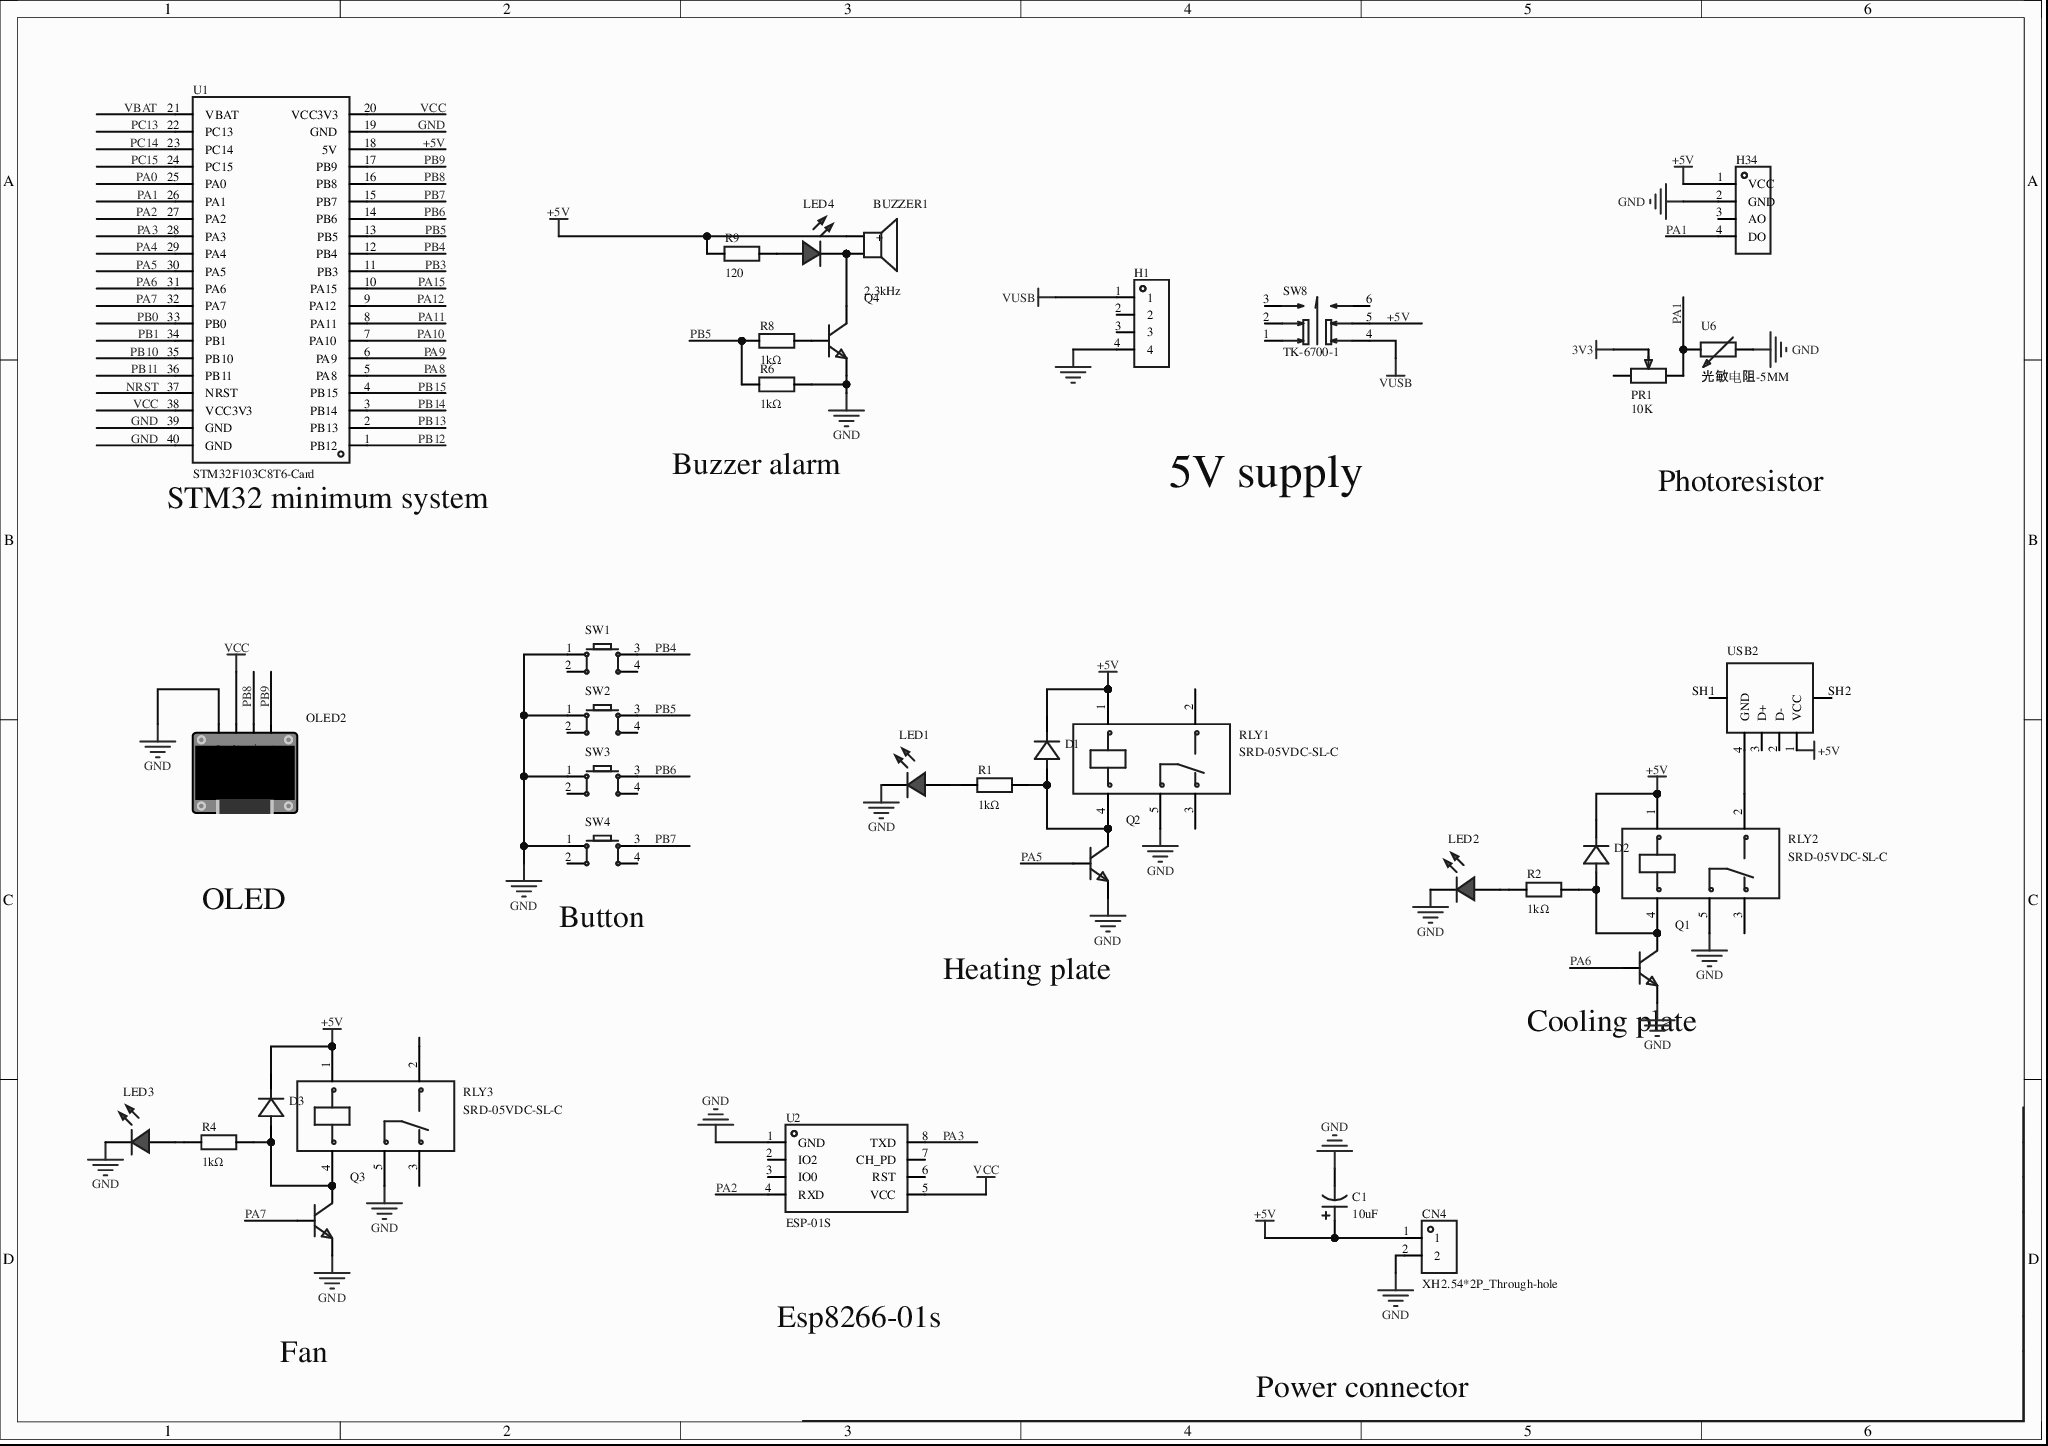
[diagram p0: MISC51908-3.schdoc]
# Altium project MISC51908-2.PrjPcb
1 sheet, 36 parts. Net scope: global (net labels, ports and power ports of the same name join across sheets).
Board file: MISC51908.pcbdoc

## Sheet MISC51908-3.schdoc
size 297 x 209 mm; Version: V1.0; @Project Name: MISC51908; @Page Count: 1; @Update Date: 2026-05-05; @Create Date: 2026-05-05; @Schematic Name: MISC51908; @Page No: 1; @Create Time: 23:22:16; @Update Time: 17:32:40; @Board Name: MISC51908

### Parts
BUZZER1  2.3kHz  [BUZ-TH_BD12.0-P7.60-D0.6-FD]
C1  10uF  [CAP-TH_BD5.0-P2.00-D0.8-FD-10UF50VC110GL]
CN4  XH2.54*2P_Through-hole  [CONN-TH_2P-P2.50-XH2.54-2P]
D1  (no value)  [DO_1N4007]
D2  (no value)  [DO_1N4007]
D3  (no value)  [DO_1N4007]
H1  (no value)  [HDR-TH_4P-P2.54-V-F]
H34  (no value)  [HDR-TH_4P-P2.54-V-F]
LED1  (no value)  [LED_TH-3mm]
LED2  (no value)  [LED_TH-3mm]
LED3  (no value)  [LED_TH-3mm]
LED4  (no value)  [LED_TH-3mm]
OLED2  (no value)  [0.96OLED_4P]
PR1  10K  [R_3386P]
Q1  (no value)  [S8050_TO_92]
Q2  (no value)  [S8050_TO_92]
Q3  (no value)  [S8050_TO_92]
Q4  (no value)  [S8050_TO_92]
R1  1kΩ  [Res_1/4W]
R2  1kΩ  [Res_1/4W]
R4  1kΩ  [Res_1/4W]
R6  1kΩ  [Res_1/4W]
R8  1kΩ  [Res_1/4W]
R9  120  [Res_1/4W]
RLY1  SRD-05VDC-SL-C  [RELAY-TH_SRD-XXVDC-XL-C]
RLY2  SRD-05VDC-SL-C  [RELAY-TH_SRD-XXVDC-XL-C]
RLY3  SRD-05VDC-SL-C  [RELAY-TH_SRD-XXVDC-XL-C]
SW1  (no value)  [SW-TH_4P-L6.0-W6.0-P4.50-LS6.5]
SW2  (no value)  [SW-TH_4P-L6.0-W6.0-P4.50-LS6.5]
SW3  (no value)  [SW-TH_4P-L6.0-W6.0-P4.50-LS6.5]
SW4  (no value)  [SW-TH_4P-L6.0-W6.0-P4.50-LS6.5]
SW8  TK-6700-1  [SW-TH_TK-6700-1]
U1  STM32F103C8T6-Card  [CONN-TH_L53.3-W22.9_STM32F103C8T6-CARD]
U2  ESP-01S  [WIFIM-TH_ESP-01S]
U6  光敏电阻-5MM  [RES-TH_L4.9-W4.3-P3.4]
USB2  (no value)  [USB_ Type-A]

### Nets
3V3: PR1.2
+5V: BUZZER1.1(+) C1.1 CN4.1 D1.1(K) D2.1(K) D3.1(K) H34.1(VCC) R9.1 RLY1.1 RLY2.1 RLY3.1 SW8.5 U1.18(5V) USB2.1(VCC)
GND: C1.2 CN4.2 H1.4 H34.2(GND) LED1.2(A) LED2.2(A) LED3.2(A) OLED2.1(GND) Q1.1(E) Q2.1(E) Q3.1(E) Q4.1(E) R6.2 RLY1.5 RLY2.5 RLY3.5 SW1.1 SW2.1 SW3.1 SW4.1 U1.19(GND) U1.39(GND) U1.40(GND) U2.1(GND) U6.1
VCC: OLED2.2(VCC) U1.20(VCC3V3) U1.38(VCC3V3) U2.5(VCC)
VUSB: H1.1 SW8.4
NRST: U1.37(NRST)
PA0: U1.25(PA0)
PA1: H34.4(DO) PR1.1 U1.26(PA1) U6.2
PA2: U1.27(PA2) U2.4(RXD)
PA3: U1.28(PA3) U2.8(TXD)
PA4: U1.29(PA4)
PA5: Q2.2(B) U1.30(PA5)
PA6: Q1.2(B) U1.31(PA6)
PA7: Q3.2(B) U1.32(PA7)
PA8: U1.5(PA8)
PA9: U1.6(PA9)
PA10: U1.7(PA10)
PA11: U1.8(PA11)
PA12: U1.9(PA12)
PA15: U1.10(PA15)
PB0: U1.33(PB0)
PB1: U1.34(PB1)
PB3: U1.11(PB3)
PB4: SW1.3 U1.12(PB4)
PB5: R6.1 R8.1 SW2.3 U1.13(PB5)
PB6: SW3.3 U1.14(PB6)
PB7: SW4.3 U1.15(PB7)
PB8: OLED2.3(SCL) U1.16(PB8)
PB9: OLED2.4(SDA) U1.17(PB9)
PB10: U1.35(PB10)
PB11: U1.36(PB11)
PB12: U1.1(PB12)
PB13: U1.2(PB13)
PB14: U1.3(PB14)
PB15: U1.4(PB15)
PC13: U1.22(PC13)
PC14: U1.23(PC14)
PC15: U1.24(PC15)
VBAT: U1.21(VBAT)
NetBUZZER1_2: BUZZER1.2 LED4.2(A) Q4.3(C)
NetD1_2: D1.2(A) Q2.3(C) R1.2 RLY1.4
NetD2_2: D2.2(A) Q1.3(C) R2.2 RLY2.4
NetD3_2: D3.2(A) Q3.3(C) R4.2 RLY3.4
NetLED1_1: LED1.1(C) R1.1
NetLED2_1: LED2.1(C) R2.1
NetLED3_1: LED3.1(C) R4.1
NetLED4_1: LED4.1(C) R9.2
NetQ4_2: Q4.2(B) R8.2
NetRLY2_2: RLY2.2 USB2.4(GND)

Not connected (* = marked no-connect by the designer): H1 2 3; H34 3(AO); PR1 3; RLY1 2 3; RLY2 3; RLY3 2 3; SW1 2 4; SW2 2 4; SW3 2 4; SW4 2 4; SW8 1* 2* 3* 6*; U2 2(IO2)* 3(IO0)* 6(RST)* 7(CH_PD)*; USB2 2(D-) 3(D+) SH1 SH2

### Notes on the sheet
- (near U1) STM32 minimum system
- Buzzer alarm
- 5V supply
- Photoresistor
- OLED
- (near SW4) Button
- Heating plate
- (near Q1) Cooling plate
- Fan
- Esp8266-01s
- Power connector

### Library data of the parts
BUZZER1 = TMB12A05_C96093: Drive mode:Active (built-in driver circuit);Construction type:Electromagnetic;Rated voltage:5V;Frequency:2.3kHz;Sound pressure (SPL):85dB@5V,10cm;; Manufacturer: 华能; 3D Model: 16ab50e14c5b4f2c986c135bdba60e37; 3D Model Transform: 472.44,472.176,0,90,0,0,-0.787,0,-177.165; Rated Voltage: 5V; Operating Voltage: 4V~8V; AddInBom: yes; ModelName: BUZ-TH_D12.0-H9.5-P7.60; Symbol: TMB12A05; Device: TMB12A05_C96093; LCSC Part Name: TMB12A05; Supplier Part: C96093; Manufacturer Part: TMB12A05; Supplier Footprint: 插件,D=12mm; JLCPCB Part Class: Extended Part; Datasheet: https://atta.szlcsc.com/upload/public/pdf/source/20170522/1495448324811.pdf; Supplier: LCSC; Oscillator Circuit: Active (built-in driver circuit); Technology Type: Electromagnetic; Value: 2.3kHz; Sound Pressure Level (SPL): 85dB@5V,10cm; Diameter (φD): 12mm; Height: 9.8mm; ConvertToPcb: yes; FootprintName: BUZ-TH_BD12.0-P7.60-D0.6-FD
C1 = 10UF50VC110GL: Capacitance:10uF;Tolerance:±20%;Rated voltage:50V;Ripple current:120mA@100KHz;Equivalent series resistance (ESR):1.6Ω;; Manufacturer: Econd(米朗电子); AddInBom: yes; Tolerance: ±20%; Voltage Rating: 50V; Equivalent Series Resistance(ESR): 1.6Ω; Pin Spacing: 2mm; Lifetime: 5000hrs@105℃; Symbol: 10UF50VC110GL; Device: 10UF50VC110GL; LCSC Part Name: 10uF ±20% 50V; SupplierPart: C46867109; ManufacturerPart: 10UF50VC110GL; Supplier Footprint: 插件,D5xL11mm; JLCPCB Part Class: Extended Part; Datasheet: https://item.szlcsc.com/datasheet/10UF50VC110GL/49031974.html; Supplier: LCSC; ConvertToPcb: yes; FootprintName: CAP-TH_BD5.0-P2.00-D0.8-FD-10UF50VC110GL; Value: 10uF; Ripple Current: 120mA@100KHz; Diameter: 5mm; Height - Seated (Max): 11mm; Operating Temperature: -40℃~+105℃
CN4 = XH2.54*2P_直插: 3D Model: 325c595e30db4df8abe76612dd40b0fa0819f05c4eef4c71ace90d822a990e87; 3D Model Transform: 295.275,228.346,0,180,0,0,-0.002,-20.079,-137.795; AddInBom: yes; Device: XH2.54*2P_Through-hole; Symbol: XH2.54*2P_Through-hole; LCSC Part Name: XH2.54*2P_直插; Supplier Part: C9900008615; Manufacturer Part: XH2.54*2P_直插; Supplier Footprint: XH2.54_2P; JLCPCB Part Class: Extended Part; Supplier: LCSC; FootprintName: CONN-TH_2P-P2.50-XH2.54-2P; ConvertToPcb: yes; ModelName: CONN-TH_2P-P2.50-XH2.54-2P
D1-D3 = D_1N4007A: AddInBom: yes; ModelId: 6de1e9b71a0d4751b4e9df530304c1a30819f05c4eef4c71ace90d822a990e87; ModelName: DO-41_D2.4-L4.7-P8.70; ModelTransform: 373.9,94.4,232.29,0,0,0,0,0,-140; Symbol: D_1N4007; Device: D_1N4007A; Supplier Footprint: DO-41; ConvertToPcb: yes; FootprintName: DO_1N4007
H1 = HDR-F_2.54_1x4P: Symbol: 2.54-1*4P female; ConvertToPcb: yes; ModelId: d187812051054f85879fcaa51a310d8e0819f05c4eef4c71ace90d822a990e87; ModelTransform: 419.6842,98.464,0,0,0,0,0,0,-118.11; Device: HDR-F_2.54_1x4P; AddInBom: yes; SupplierPart: C2718488; Supplier Footprint: 插件; FootprintName: HDR-TH_4P-P2.54-V-F; ModelName: HDR-TH_4P-P2.54-V-F
H34 = HDR-F_2.54_1x4P: Symbol: 2.54-1*4P female_1; 3D Model: d187812051054f85879fcaa51a310d8e0819f05c4eef4c71ace90d822a990e87; 3D Model Transform: 419.6842,98.464,0,0,0,0,0,0,-118.11; ConvertToPcb: yes; Device: HDR-F_2.54_1x4P; Supplier Part: C2718488; Supplier Footprint: 插件; AddInBom: yes; FootprintName: HDR-TH_4P-P2.54-V-F; ModelName: HDR-TH_4P-P2.54-V-F
LED1-LED4 = LED_TH-R_3mm: 3D Model: a497c992633541038a38947cdc58012f0819f05c4eef4c71ace90d822a990e87; 3D Model Transform: 141.274,153.327,0,0,0,0,-5.984,0,-137.795; ConvertToPcb: yes; ModelName: LED-TH-3mm_R; Symbol: LED_TH-R; Device: LED_TH-R_3mm; Supplier Footprint: 插件; AddInBom: yes; FootprintName: LED_TH-3mm
OLED2 = 0.96OLED模块_4P: Symbol: 0.96OLED module_4P; ConvertToPcb: yes; ModelId: 79c000fdb68d45a296c2e9bedf4f9055; ModelTransform: 1393.69792,1318.895,0,0,0,0,0,-560.079,-137.795; Device: 0.96OLED module_4P; AddInBom: yes; FootprintName: 0.96OLED_4P; Supplier Footprint: 插件; ModelName: 0.96OLED_4P
PR1 = R_3386P: Symbol: 3386P-1-103LF; ConvertToPcb: yes; ModelId: 6a25d8a4450b4318959c1cd98efa6b0c0819f05c4eef4c71ace90d822a990e87; ModelName: RES-ADJ-TH_3P-L9.5-W9.5-P2.54-BR-BS; ModelTransform: 375.19,375.19,387,-90,0,0,0,0,-197; Device: R_3386P; AddInBom: yes; FootprintName: R_3386P; Value: 10K; Supplier Footprint: 直插
Q1-Q4 = S8050_TO_NPN: 3D Model: aafe8e06f2154e7c93506efd0d6632dd; 3D Model Transform: 180.78,141.44,417.3,0,0,0,0,0,-200; ConvertToPcb: yes; ModelName: TO-92-3_L4.9-W3.7-P1.27-L; Symbol: S8050_TO_NPN; Device: S8050_TO_NPN; Supplier Footprint: TO-92; AddInBom: yes; FootprintName: S8050_TO_92
R1 R2 R4 = Res_AXIAL-1/8W: Symbol: Resistor; 3D Model: b2b5ae7ae4c642178fe0039925c86a3f0819f05c4eef4c71ace90d822a990e87; 3D Model Transform: 282.86,66.88,253.09,0,0,0,0,0,-191; ConvertToPcb: yes; ModelName: RES-TH_BD1.8-L3.2-P7.20-D0.4; Device: Res_AXIAL-1/8W; Supplier Footprint: 轴向引线; Value: 1kΩ; AddInBom: yes; FootprintName: Res_1/4W
R6 R8 R9 = Res_AXIAL-1/4W: Symbol: Resistor; 3D Model: 463263665006444ab7a47bd11b0cf956; 3D Model Transform: 427.165,94.32816,0,0,0,0,0,0,-196.85; AddInBom: yes; ModelName: RES-TH_BD2.4-L6.3-P10.30-D0.6; Device: Res_AXIAL-1/4W; Supplier Footprint: 轴向引线; ConvertToPcb: yes; FootprintName: Res_1/4W
  R6 R8: Value: 1kΩ
  R9: Value: 120
RLY1-RLY3 = SRD-05VDC-SL-C: 线圈电压:5V;触点形式:一组转换:1C(单刀双掷-转换);触点容量(电阻负载):-;最大切换电压:250V@AC;最大切换电流:15A;; Manufacturer: 松乐; 3D Model: d0eda9b8bf8746d18ae810ab88dc78e70819f05c4eef4c71ace90d822a990e87; 3D Model Transform: 755.904,622.4397,0,0,0,0,34.882,0,-118.11; Coil Voltage: 5V; Coil Rated Power: 360mW; Switching Current(Max): 15A; Coil Type: Non-polar, single coil; Coil Resistance: 70Ω; Contact Resistance: 100mΩ; Operate Time: 10ms; AddInBom: yes; ModelName: RELAY-TH_L19.2-W15.6-H15.8; Symbol: SRD-05VDC-SL-C; Device: SRD-05VDC-SL-C; LCSC Part Name: 蓝色 单组转换型继电器; Supplier Part: C35449; Manufacturer Part: SRD-05VDC-SL-C; Supplier Footprint: 插件,19.2x15.6mm; JLCPCB Part Class: Extended Part; Datasheet: https://item.szlcsc.com/datasheet/SRD-05VDC-SL-C/36422.html; Supplier: LCSC; Contact Form: 一组转换:1C(单刀双掷-转换); Number of Pins: 5; Contact Rating: -; Switching Voltage(Max): 250V@AC; Release Time: 10ms; ConvertToPcb: yes; FootprintName: RELAY-TH_SRD-XXVDC-XL-C
SW1 = Key_TH_6x6x6: Contact current:50mA;Rated voltage (DC):12V;Insulation resistance:100MΩ;Circuit structure:SPST;Mounting:Through-hole;Button shape:Round button;Button/cap colour:Black;Actuation force:260gf@±30gf;Operating temperature:-25℃~+70℃;Pin style:PC pin;Switch length:6mm;Switch width:6mm;Switch height:6mm;With bracket:No;; Symbol: Tact switch; 3D Model: 20eee248bc684ccd8cbdbb1d0d91ec6f0819f05c4eef4c71ace90d822a990e87; 3D Model Transform: 236.22,323.03,0,90,0,0,0,0,-137.795; AddInBom: yes; ModelName: SW-TH_4P-L6.0-W6.0-H5.0-LS6.5-P4.50; Device: Key_TH_6x6x6; Supplier Footprint: 插件; FootprintName: SW-TH_4P-L6.0-W6.0-P4.50-LS6.5; ConvertToPcb: yes
SW2-SW4 = Key_TH_6x6x6: Contact current:50mA;Rated voltage (DC):12V;Insulation resistance:100MΩ;Circuit structure:SPST;Mounting:Through-hole;Button shape:Round button;Button/cap colour:Black;Actuation force:260gf@±30gf;Operating temperature:-25℃~+70℃;Pin style:PC pin;Switch length:6mm;Switch width:6mm;Switch height:6mm;With bracket:No;; Symbol: Tact switch; AddInBom: yes; ModelId: 20eee248bc684ccd8cbdbb1d0d91ec6f0819f05c4eef4c71ace90d822a990e87; ModelName: SW-TH_4P-L6.0-W6.0-H5.0-LS6.5-P4.50; ModelTransform: 236.22,323.03,0,90,0,0,0,0,-137.795; Device: Key_TH_6x6x6; FootprintName: SW-TH_4P-L6.0-W6.0-P4.50-LS6.5; ConvertToPcb: yes; Supplier Footprint: 插件
SW8 = TK-6700-1: Manufacturer: Yuandi(元迪); 3D Model: 1dccfbf2ceb24a728093c1f6ee61932a; 3D Model Transform: 275.59,275.59,0,90,0,0,0,0,-137.795; AddInBom: yes; Symbol: TK-6700-1; Device: TK-6700-1; LCSC Part Name: 自锁开关7*7*12.7有声有锁高导高柄插件双排6P按键开关带锁DIP六脚; Supplier Part: C528782; Manufacturer Part: TK-6700-1; Supplier Footprint: 插件; JLCPCB Part Class: Extended Part; Datasheet: https://atta.szlcsc.com/upload/public/pdf/source/20200831/C528782_58F076EBF84BD8A9E2DE38DB1C0986D4.pdf; Supplier: LCSC; ConvertToPcb: yes; FootprintName: SW-TH_TK-6700-1; ModelName: SW-TH_TK-6700-1
U1 = STM32F103C8T6-Card: AddInBom: yes; Device: STM32F103C8T6-Card; Symbol: STM32F103C8T6-CARD; FootprintName: CONN-TH_L53.3-W22.9_STM32F103C8T6-CARD; LCSC Part Name: STM32F103C8T6-Card; SupplierPart: C9900077949; ManufacturerPart: STM32F103C8T6-Card; Supplier Footprint: 插件; Supplier: LCSC; ConvertToPcb: yes
U2 = ESP-01S_C111009: 3D Model: eb7175da78ae48b3b1568cfe3027405f0819f05c4eef4c71ace90d822a990e87; 3D Model Transform: 582.676,976.37608,0,0,0,0,0,388.346,-118.11; AddInBom: yes; Symbol: ESP-01S; Device: ESP-01S_C111009; LCSC Part Name: ESP-01S; Supplier Part: C111009; Manufacturer Part: ESP-01S; Supplier Footprint: -; JLCPCB Part Class: Extended Part; Supplier: LCSC; ConvertToPcb: yes; FootprintName: WIFIM-TH_ESP-01S; ModelName: WIFIM-TH_ESP-01S
U6 = 光敏电阻-5MM: 3D Model: 8cda4899688949e78503a56fe341541c0819f05c4eef4c71ace90d822a990e87; 3D Model Transform: 169.291,200.6107,0,90,0,0,0,0,-196.85; AddInBom: yes; Symbol: 光敏电阻-5MM; Device: 光敏电阻-5MM; LCSC Part Name: 光敏电阻-5MM; Supplier Part: C9900003115; Manufacturer Part: 光敏电阻-5MM; Supplier Footprint: RES-TH_4.3X4.9X3.37P; JLCPCB Part Class: Extended Part; Supplier: LCSC; ConvertToPcb: yes; FootprintName: RES-TH_L4.9-W4.3-P3.4; ModelName: RES-TH_L4.9-W4.3-P3.4
USB2 = USB_ Type-A: AddInBom: yes; ModelId: 0a0bfc60af8549fa93b7465d8aaf02b10819f05c4eef4c71ace90d822a990e87; ModelName: USB-A-TH__USB-AF-90; ModelTransform: 612.05,551.18,446.85,0,0,0,0,-15.75,-157.48; Symbol: USB_Type-A; Device: USB_ Type-A; ConvertToPcb: yes; FootprintName: USB_ Type-A; Supplier Footprint: 插件